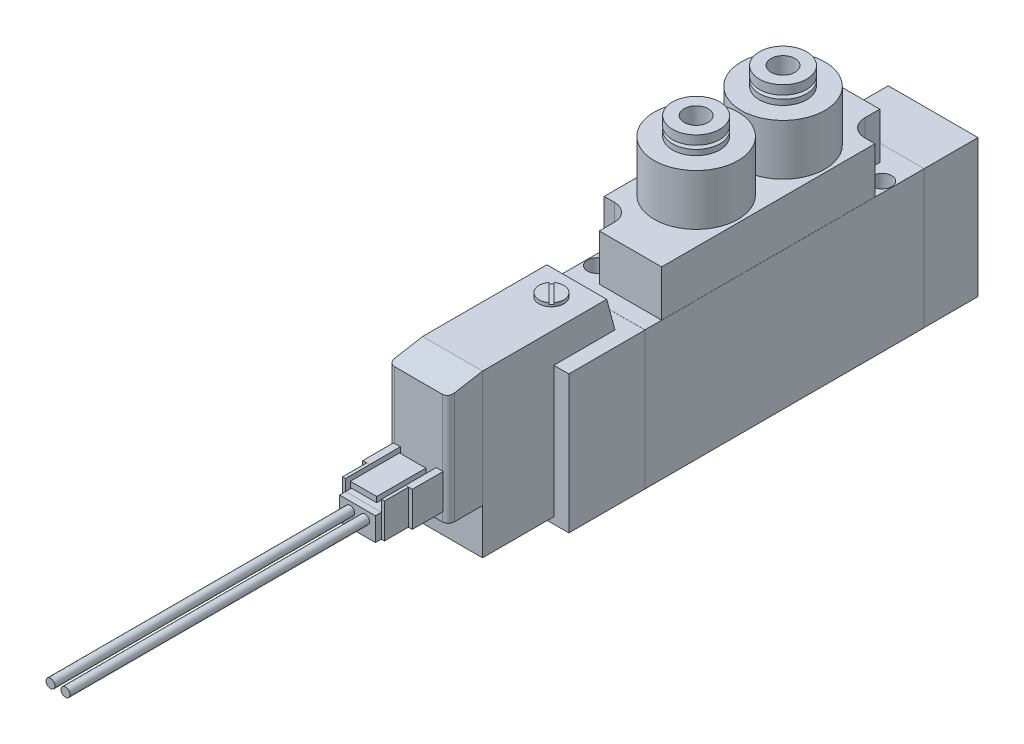
SolidWorks part; units mm, degrees
ref_plane "前视" through (0, 0, 0) normal (0, 0, 1) x (1, 0, 0)
ref_plane "上视" through (0, 0, 0) normal (0, 1, 0) x (1, 0, 0)
ref_plane "右视" through (0, 0, 0) normal (1, 0, 0) x (0, 0, -1)
sketch "草图1" plane through (0, 0, 0) normal (1, 0, 0) x (0, 0, -1)
  line L0 (0, 0) -> (46.6, 0)
  line L1 (46.6, 0) -> (46.6, 23)
  line L2 (46.6, 23) -> (0, 23)
  line L3 (0, 23) -> (0, 0)
extrude "拉伸1" add sketch "草图1" against normal blind 15
ref_plane "基准面1" through (0, 0, -46.6) normal (0, 0, -1) x (-1, 0, 0)
sketch "草图2" plane through (0, 0, -46.6) normal (0, 0, -1) x (-1, 0, 0)
  line L0 (0.01, 22.99) -> (0.01, 0.01)
  line L1 (0.01, 0.01) -> (14.99, 0.01)
  line L2 (14.99, 0.01) -> (14.99, 22.99)
  line L3 (14.99, 22.99) -> (0.01, 22.99)
ref_plane "基准面2" through (0, 0, -46.6) normal (0, 0, -1) x (-1, 0, 0)
sketch "草图3" plane through (0, 0, -46.6) normal (0, 0, -1) x (-1, 0, 0)
  line L0 (0.01, 22.99) -> (0.01, 0.01)
  line L1 (0.01, 0.01) -> (14.99, 0.01)
  line L2 (14.99, 0.01) -> (14.99, 22.99)
  line L3 (14.99, 22.99) -> (0.01, 22.99)
extrude "拉伸2" add sketch "草图2" along normal blind 9
extrude "拉伸3" add sketch "草图3" against normal blind 0.01
ref_plane "基准面3" through (-7.5, 0, 0) normal (1, 0, 0) x (0, 0, -1)
sketch "草图4" plane through (-7.5, 0, 0) normal (1, 0, 0) x (0, 0, -1)
  line L0 (23.3, 8) -> (27.585, 8)
  line L1 (27.585, 8) -> (27.585, 0.5)
  line L2 (27.585, 0.5) -> (28.585, -0.5)
  line L3 (28.585, -0.5) -> (23.3, -0.5)
  line L4 (23.3, -0.5) -> (23.3, 8)
  line L5 (23.3, -0.5) -> (23.3, 8) construction
revolve "切除-旋转1" cut sketch "草图4" angle 360 about L5
cosmetic thread "装饰螺纹线1" parameters "D1"=5.5, "D2"=9.73
ref_plane "基准面4" through (-6.7, 0, 0) normal (1, 0, 0) x (0, 0, -1)
sketch "草图5" plane through (-6.7, 0, 0) normal (1, 0, 0) x (0, 0, -1)
  line L0 (9.7, 8) -> (13.985, 8)
  line L1 (13.985, 8) -> (13.985, 0.5)
  line L2 (13.985, 0.5) -> (14.985, -0.5)
  line L3 (14.985, -0.5) -> (9.7, -0.5)
  line L4 (9.7, -0.5) -> (9.7, 8)
  line L5 (9.7, -0.5) -> (9.7, 8) construction
revolve "切除-旋转2" cut sketch "草图5" angle 360 about L5
cosmetic thread "装饰螺纹线2" parameters "D1"=5.5, "D2"=9.73
ref_plane "基准面5" through (-8.3, 0, 0) normal (1, 0, 0) x (0, 0, -1)
sketch "草图6" plane through (-8.3, 0, 0) normal (1, 0, 0) x (0, 0, -1)
  line L0 (36.9, 8) -> (41.185, 8)
  line L1 (41.185, 8) -> (41.185, 0.5)
  line L2 (41.185, 0.5) -> (42.185, -0.5)
  line L3 (42.185, -0.5) -> (36.9, -0.5)
  line L4 (36.9, -0.5) -> (36.9, 8)
  line L5 (36.9, -0.5) -> (36.9, 8) construction
revolve "切除-旋转3" cut sketch "草图6" angle 360 about L5
cosmetic thread "装饰螺纹线3" parameters "D1"=5.5, "D2"=9.73
sketch "草图7" plane through (0, 0, 0) normal (1, 0, 0) x (0, 0, -1)
  line L0 (-12.7, 0.01) -> (0.01, 0.01)
  line L1 (0.01, 0.01) -> (0.01, 22.99)
  line L2 (0.01, 22.99) -> (-12.7, 22.99)
  line L3 (-12.7, 22.99) -> (-12.7, 0.01)
sketch "草图8" plane through (0, 0, 0) normal (1, 0, 0) x (0, 0, -1)
  line L0 (-12.7, 0.01) -> (0.01, 0.01)
  line L1 (0.01, 0.01) -> (0.01, 22.99)
  line L2 (0.01, 22.99) -> (-12.7, 22.99)
  line L3 (-12.7, 22.99) -> (-12.7, 0.01)
extrude "拉伸4" add sketch "草图7" along normal blind 0.01
extrude "拉伸5" add sketch "草图8" against normal blind 15.01
sketch "草图9" plane through (-7.5, 0, 0) normal (1, 0, 0) x (0, 0, -1)
  line L0 (-24.6, 1.1) -> (-12.7, 1.1)
  line L1 (-12.7, 1.1) -> (-12.7, 0.01)
  line L2 (-12.7, 0.01) -> (-2.5, 0.01)
  line L3 (-2.5, 0.01) -> (-2.5, 23)
  line L4 (-2.5, 23) -> (-3.8665, 28.1)
  line L5 (-3.8665, 28.1) -> (-24.6, 28.1)
  line L6 (-24.6, 28.1) -> (-24.6, 1.1)
extrude "拉伸6" add sketch "草图9" against normal blind 5 and the other way blind 5
ref_plane "基准面6" through (0, 28.1, 0) normal (0, 1, 0) x (-1, 0, 0)
sketch "草图10" plane through (0, 28.1, 0) normal (0, 1, 0) x (-1, 0, 0)
  line L0 (12.49, 24.59) -> (12.49, 29.3)
  line L1 (11.49, 30.3) -> (3.51, 30.3)
  line L2 (2.51, 29.3) -> (2.51, 24.59)
  line L3 (2.51, 24.59) -> (12.49, 24.59)
  arc A0 (12.49, 29.3) -> (11.49, 30.3) centre (11.49, 29.3) ccw
  arc A1 (3.51, 30.3) -> (2.51, 29.3) centre (3.51, 29.3) ccw
extrude "拉伸7" add sketch "草图10" against normal blind 19.45
sketch "草图11" plane through (0, 0, 0) normal (1, 0, 0) x (0, 0, -1)
  line L0 (-34.6, 26.3367) -> (-13.2574, 30.1)
  line L1 (-13.2574, 30.1) -> (-34.6, 30.1)
  line L2 (-34.6, 30.1) -> (-34.6, 26.3367)
extrude "切除-拉伸1" cut sketch "草图11" against normal blind 15
ref_plane "基准面7" through (0, 0, 30.3) normal (0, 0, 1) x (1, 0, 0)
sketch "草图12" plane through (0, 0, 30.3) normal (0, 0, 1) x (1, 0, 0)
  line L0 (-3.37, 10.2) -> (-3.37, 16)
  line L1 (-3.37, 16) -> (-4.51, 16)
  line L2 (-4.51, 16) -> (-4.51, 14.1)
  line L3 (-4.51, 14.1) -> (-10.51, 14.1)
  line L4 (-10.51, 14.1) -> (-10.51, 16)
  line L5 (-10.51, 16) -> (-11.65, 16)
  line L6 (-11.65, 16) -> (-11.65, 10.2)
  line L7 (-11.65, 10.2) -> (-3.37, 10.2)
  line L8 (-4.51, 11.34) -> (-4.51, 13.6)
  line L9 (-4.51, 13.6) -> (-10.51, 13.6)
  line L10 (-10.51, 13.6) -> (-10.51, 11.34)
  line L11 (-10.51, 11.34) -> (-4.51, 11.34)
ref_plane "基准面8" through (0, 0, 30.3) normal (0, 0, 1) x (1, 0, 0)
sketch "草图13" plane through (0, 0, 30.3) normal (0, 0, 1) x (1, 0, 0)
  line L0 (-3.37, 10.2) -> (-3.37, 16)
  line L1 (-3.37, 16) -> (-4.51, 16)
  line L2 (-4.51, 16) -> (-4.51, 14.1)
  line L3 (-4.51, 14.1) -> (-10.51, 14.1)
  line L4 (-10.51, 14.1) -> (-10.51, 16)
  line L5 (-10.51, 16) -> (-11.65, 16)
  line L6 (-11.65, 16) -> (-11.65, 10.2)
  line L7 (-11.65, 10.2) -> (-3.37, 10.2)
  line L8 (-4.51, 11.34) -> (-4.51, 13.6)
  line L9 (-4.51, 13.6) -> (-10.51, 13.6)
  line L10 (-10.51, 13.6) -> (-10.51, 11.34)
  line L11 (-10.51, 11.34) -> (-4.51, 11.34)
extrude "拉伸8" add sketch "草图12" along normal blind 5.15
extrude "拉伸9" add sketch "草图13" against normal blind 0.01
ref_plane "基准面9" through (0, 0, 35.45) normal (0, 0, 1) x (1, 0, 0)
sketch "草图14" plane through (0, 0, 35.45) normal (0, 0, 1) x (1, 0, 0)
  line L0 (-11.01, 15.99) -> (-11.01, 10.21)
  line L1 (-11.01, 10.21) -> (-4.01, 10.21)
  line L2 (-4.01, 10.21) -> (-4.01, 15.99)
  line L3 (-4.01, 15.99) -> (-4.51, 15.99)
  line L4 (-4.51, 15.99) -> (-4.51, 14.09)
  line L5 (-4.51, 14.09) -> (-10.51, 14.09)
  line L6 (-10.51, 14.09) -> (-10.51, 15.99)
  line L7 (-10.51, 15.99) -> (-11.01, 15.99)
ref_plane "基准面10" through (0, 0, 35.45) normal (0, 0, 1) x (1, 0, 0)
sketch "草图15" plane through (0, 0, 35.45) normal (0, 0, 1) x (1, 0, 0)
  line L0 (-11.01, 15.99) -> (-11.01, 10.21)
  line L1 (-11.01, 10.21) -> (-4.01, 10.21)
  line L2 (-4.01, 10.21) -> (-4.01, 15.99)
  line L3 (-4.01, 15.99) -> (-4.51, 15.99)
  line L4 (-4.51, 15.99) -> (-4.51, 14.09)
  line L5 (-4.51, 14.09) -> (-10.51, 14.09)
  line L6 (-10.51, 14.09) -> (-10.51, 15.99)
  line L7 (-10.51, 15.99) -> (-11.01, 15.99)
extrude "拉伸10" add sketch "草图14" along normal blind 4
extrude "拉伸11" add sketch "草图15" against normal blind 6
ref_plane "基准面11" through (0, 14.09, 0) normal (0, 1, 0) x (-1, 0, 0)
sketch "草图16" plane through (0, 14.09, 0) normal (0, 1, 0) x (-1, 0, 0)
  line L0 (5.71, 35.95) -> (5.71, 36.35)
  line L1 (5.71, 36.35) -> (5.31, 36.35)
  line L2 (5.31, 36.35) -> (5.31, 35.95)
  line L3 (5.31, 35.95) -> (5.71, 35.95)
ref_plane "基准面12" through (0, 14.09, 0) normal (0, 1, 0) x (-1, 0, 0)
sketch "草图17" plane through (0, 14.09, 0) normal (0, 1, 0) x (-1, 0, 0)
  line L0 (5.71, 35.95) -> (5.71, 36.35)
  line L1 (5.71, 36.35) -> (5.31, 36.35)
  line L2 (5.31, 36.35) -> (5.31, 35.95)
  line L3 (5.31, 35.95) -> (5.71, 35.95)
extrude "拉伸12" add sketch "草图16" along normal blind 1.5
extrude "拉伸13" add sketch "草图17" against normal blind 0.01
ref_plane "基准面13" through (0, 14.09, 0) normal (0, 1, 0) x (-1, 0, 0)
sketch "草图18" plane through (0, 14.09, 0) normal (0, 1, 0) x (-1, 0, 0)
  line L0 (9.71, 35.95) -> (9.71, 36.35)
  line L1 (9.71, 36.35) -> (9.31, 36.35)
  line L2 (9.31, 36.35) -> (9.31, 35.95)
  line L3 (9.31, 35.95) -> (9.71, 35.95)
ref_plane "基准面14" through (0, 14.09, 0) normal (0, 1, 0) x (-1, 0, 0)
sketch "草图19" plane through (0, 14.09, 0) normal (0, 1, 0) x (-1, 0, 0)
  line L0 (9.71, 35.95) -> (9.71, 36.35)
  line L1 (9.71, 36.35) -> (9.31, 36.35)
  line L2 (9.31, 36.35) -> (9.31, 35.95)
  line L3 (9.31, 35.95) -> (9.71, 35.95)
extrude "拉伸14" add sketch "草图18" along normal blind 1.5
extrude "拉伸15" add sketch "草图19" against normal blind 0.01
ref_plane "基准面15" through (0, 15.99, 0) normal (0, 1, 0) x (-1, 0, 0)
sketch "草图20" plane through (0, 15.99, 0) normal (0, 1, 0) x (-1, 0, 0)
  line L0 (9.71, 39.45) -> (5.31, 39.45)
  line L1 (5.31, 39.45) -> (5.31, 31.25)
  line L2 (5.31, 31.25) -> (9.71, 31.25)
  line L3 (9.71, 31.25) -> (9.71, 39.45)
extrude "拉伸16" add sketch "草图20" against normal blind 0.9
ref_plane "基准面16" through (0, 0, 39.45) normal (0, 0, 1) x (1, 0, 0)
sketch "草图21" plane through (0, 0, 39.45) normal (0, 0, 1) x (1, 0, 0)
  line L0 (-4.52, 10.22) -> (-4.52, 14.1)
  line L1 (-4.52, 14.1) -> (-10.5, 14.1)
  line L2 (-10.5, 14.1) -> (-10.5, 10.22)
  line L3 (-10.5, 10.22) -> (-4.52, 10.22)
ref_plane "基准面17" through (0, 0, 39.45) normal (0, 0, 1) x (1, 0, 0)
sketch "草图22" plane through (0, 0, 39.45) normal (0, 0, 1) x (1, 0, 0)
  line L0 (-4.52, 10.22) -> (-4.52, 14.1)
  line L1 (-4.52, 14.1) -> (-10.5, 14.1)
  line L2 (-10.5, 14.1) -> (-10.5, 10.22)
  line L3 (-10.5, 10.22) -> (-4.52, 10.22)
extrude "拉伸17" add sketch "草图21" along normal blind 1
extrude "拉伸18" add sketch "草图22" against normal blind 0.01
ref_plane "基准面18" through (0, 0, 40.45) normal (0, 0, 1) x (1, 0, 0)
sketch "草图23" plane through (0, 0, 40.45) normal (0, 0, 1) x (1, 0, 0)
  circle A0 centre (-8.75, 12.75) radius 0.75
ref_plane "基准面19" through (0, 0, 40.45) normal (0, 0, 1) x (1, 0, 0)
sketch "草图24" plane through (0, 0, 40.45) normal (0, 0, 1) x (1, 0, 0)
  circle A0 centre (-8.75, 12.75) radius 0.75
extrude "拉伸19" add sketch "草图23" along normal blind 50
extrude "拉伸20" add sketch "草图24" against normal blind 0.01
ref_plane "基准面20" through (0, 0, 40.45) normal (0, 0, 1) x (1, 0, 0)
sketch "草图25" plane through (0, 0, 40.45) normal (0, 0, 1) x (1, 0, 0)
  circle A0 centre (-6.25, 12.75) radius 0.75
ref_plane "基准面21" through (0, 0, 40.45) normal (0, 0, 1) x (1, 0, 0)
sketch "草图26" plane through (0, 0, 40.45) normal (0, 0, 1) x (1, 0, 0)
  circle A0 centre (-6.25, 12.75) radius 0.75
extrude "拉伸21" add sketch "草图25" along normal blind 50
extrude "拉伸22" add sketch "草图26" against normal blind 0.01
ref_plane "基准面22" through (0, 28.1, 0) normal (0, 1, 0) x (-1, 0, 0)
sketch "草图27" plane through (0, 28.1, 0) normal (0, 1, 0) x (-1, 0, 0)
  circle A0 centre (7.5, 8.1) radius 2.075
ref_plane "基准面23" through (0, 28.1, 0) normal (0, 1, 0) x (-1, 0, 0)
sketch "草图28" plane through (0, 28.1, 0) normal (0, 1, 0) x (-1, 0, 0)
  circle A0 centre (7.5, 8.1) radius 2.075
extrude "拉伸23" add sketch "草图27" along normal blind 0.6
extrude "拉伸24" add sketch "草图28" against normal blind 0.01
ref_plane "基准面24" through (0, 28.7, 0) normal (0, 1, 0) x (-1, 0, 0)
sketch "草图29" plane through (0, 28.7, 0) normal (0, 1, 0) x (-1, 0, 0)
  line L0 (5.8182, 9.3576) -> (8.7576, 6.4182)
  line L1 (9.1818, 6.8424) -> (6.2424, 9.7818)
  arc A0 (6.2424, 9.7818) -> (5.8182, 9.3576) centre (7.5, 8.1) ccw
  arc A1 (8.7576, 6.4182) -> (9.1818, 6.8424) centre (7.5, 8.1) ccw
ref_plane "基准面25" through (0, 28.7, 0) normal (0, 1, 0) x (-1, 0, 0)
sketch "草图30" plane through (0, 28.7, 0) normal (0, 1, 0) x (-1, 0, 0)
  line L0 (5.8182, 9.3576) -> (8.7576, 6.4182)
  line L1 (9.1818, 6.8424) -> (6.2424, 9.7818)
  arc A0 (6.2424, 9.7818) -> (5.8182, 9.3576) centre (7.5, 8.1) ccw
  arc A1 (8.7576, 6.4182) -> (9.1818, 6.8424) centre (7.5, 8.1) ccw
extrude "切除-拉伸3" cut sketch "草图30" against normal blind 0.25
ref_plane "基准面26" through (0, 23, 0) normal (0, 1, 0) x (-1, 0, 0)
sketch "草图31" plane through (0, 23, 0) normal (0, 1, 0) x (-1, 0, 0)
  line L0 (14.99, -43.8) -> (14.99, -2.8)
  line L1 (14.99, -2.8) -> (0.01, -2.8)
  line L2 (0.01, -2.8) -> (0.01, -43.8)
  line L3 (0.01, -43.8) -> (14.99, -43.8)
sketch "草图32" plane through (0, 23, 0) normal (0, 1, 0) x (-1, 0, 0)
  line L0 (14.99, -43.8) -> (14.99, -2.8)
  line L1 (14.99, -2.8) -> (0.01, -2.8)
  line L2 (0.01, -2.8) -> (0.01, -43.8)
  line L3 (0.01, -43.8) -> (14.99, -43.8)
extrude "拉伸25" add sketch "草图31" along normal blind 7.7
extrude "拉伸26" add sketch "草图32" against normal blind 0.01
sketch "草图33" plane through (0, 23, 0) normal (0, 1, 0) x (-1, 0, 0)
  line L0 (4.6, -43.8) -> (4.6, -41.3)
  line L1 (1.7, -38.4) -> (-2, -38.4)
  line L2 (-2, -38.4) -> (-2, -43.8)
  line L3 (-2, -43.8) -> (4.6, -43.8)
  arc A0 (4.6, -41.3) -> (1.7, -38.4) centre (1.7, -41.3) ccw
extrude "切除-拉伸4" cut sketch "草图33" along normal blind 8.7
sketch "草图34" plane through (0, 23, 0) normal (0, 1, 0) x (-1, 0, 0)
  line L0 (16, -2.8) -> (10.4, -2.8)
  line L1 (10.4, -2.8) -> (10.4, -5.3)
  line L2 (13.3, -8.2) -> (16, -8.2)
  line L3 (16, -8.2) -> (16, -2.8)
  arc A0 (10.4, -5.3) -> (13.3, -8.2) centre (13.3, -5.3) ccw
extrude "切除-拉伸5" cut sketch "草图34" along normal blind 8.7
ref_plane "基准面27" through (0, 30.7, 0) normal (0, 1, 0) x (-1, 0, 0)
sketch "草图35" plane through (-7.5, 0, 0) normal (1, 0, 0) x (0, 0, -1)
  line L0 (16.05, 42.2) -> (20, 42.2)
  line L1 (20, 42.2) -> (20, 40.7)
  line L2 (20, 40.7) -> (18.25, 40.7)
  line L3 (18.25, 40.7) -> (18.25, 40.1)
  line L4 (18.25, 40.1) -> (20, 40.1)
  line L5 (20, 40.1) -> (20, 39.2)
  line L6 (20, 39.2) -> (23.05, 39.2)
  line L7 (23.05, 39.2) -> (23.05, 30.69)
  line L8 (23.05, 30.69) -> (16.05, 30.69)
  line L9 (16.05, 30.69) -> (16.05, 42.2)
  line L10 (16.05, 30.69) -> (16.05, 42.2) construction
revolve "旋转1" add sketch "草图35" angle 360 about L10
sketch "草图36" plane through (-7.5, 0, 0) normal (1, 0, 0) x (0, 0, -1)
  line L0 (30.55, 42.2) -> (34.5, 42.2)
  line L1 (34.5, 42.2) -> (34.5, 40.7)
  line L2 (34.5, 40.7) -> (32.75, 40.7)
  line L3 (32.75, 40.7) -> (32.75, 40.1)
  line L4 (32.75, 40.1) -> (34.5, 40.1)
  line L5 (34.5, 40.1) -> (34.5, 39.2)
  line L6 (34.5, 39.2) -> (37.55, 39.2)
  line L7 (37.55, 39.2) -> (37.55, 30.69)
  line L8 (37.55, 30.69) -> (30.55, 30.69)
  line L9 (30.55, 30.69) -> (30.55, 42.2)
  line L10 (30.55, 30.69) -> (30.55, 42.2) construction
revolve "旋转2" add sketch "草图36" angle 360 about L10
ref_plane "基准面28" through (0, 42.2, 0) normal (0, 1, 0) x (-1, 0, 0)
sketch "草图37" plane through (0, 42.2, 0) normal (0, 1, 0) x (-1, 0, 0)
  circle A0 centre (7.5, -16.05) radius 2
extrude "切除-拉伸6" cut sketch "草图37" against normal blind 20.2
ref_plane "基准面29" through (0, 42.2, 0) normal (0, 1, 0) x (-1, 0, 0)
sketch "草图38" plane through (0, 42.2, 0) normal (0, 1, 0) x (-1, 0, 0)
  circle A0 centre (7.5, -30.55) radius 2
extrude "切除-拉伸7" cut sketch "草图38" against normal blind 20.2
ref_plane "基准面30" through (0, 0.5, 0) normal (0, 1, 0) x (-1, 0, 0)
ref_plane "基准面31" through (0, 0.7, 0) normal (0, 1, 0) x (-1, 0, 0)
ref_plane "基准面32" through (0, 0, -45.8) normal (0, 0, 1) x (1, 0, 0)
ref_plane "基准面33" through (0, 16.7, 0) normal (0, 1, 0) x (-1, 0, 0)
sketch "草图39" plane through (0, 16.7, 0) normal (0, 1, 0) x (-1, 0, 0)
  line L0 (15.5, -34.6) -> (15.5, -36.83)
  line L1 (15.5, -36.83) -> (14.5, -35.83)
  line L2 (14.5, -35.83) -> (8.5, -35.83)
  line L3 (8.5, -35.83) -> (8.5, -34.6)
  line L4 (8.5, -34.6) -> (15.5, -34.6)
  line L5 (8.5, -34.6) -> (15.5, -34.6) construction
revolve "切除-旋转4" cut sketch "草图39" angle 360 about L5
cosmetic thread "装饰螺纹线4" parameters "D1"=5, "D2"=3
sketch "草图40" plane through (0, 16.7, 0) normal (0, 1, 0) x (-1, 0, 0)
  line L0 (15.5, -12) -> (15.5, -14.23)
  line L1 (15.5, -14.23) -> (14.5, -13.23)
  line L2 (14.5, -13.23) -> (8.5, -13.23)
  line L3 (8.5, -13.23) -> (8.5, -12)
  line L4 (8.5, -12) -> (15.5, -12)
  line L5 (8.5, -12) -> (15.5, -12) construction
revolve "切除-旋转5" cut sketch "草图40" angle 360 about L5
cosmetic thread "装饰螺纹线5" parameters "D1"=5, "D2"=3
sketch "草图41" plane through (0, 30.7, 0) normal (0, 1, 0) x (1, 0, 0)
  circle A0 centre (-13.3, 5.3) radius 1.6
  circle A1 centre (-1.7, 41.3) radius 1.6
  dimension "D1" = 3.2
  dimension "D2" = 3.2
extrude "切除-拉伸8" cut sketch "草图41" against normal blind 523
